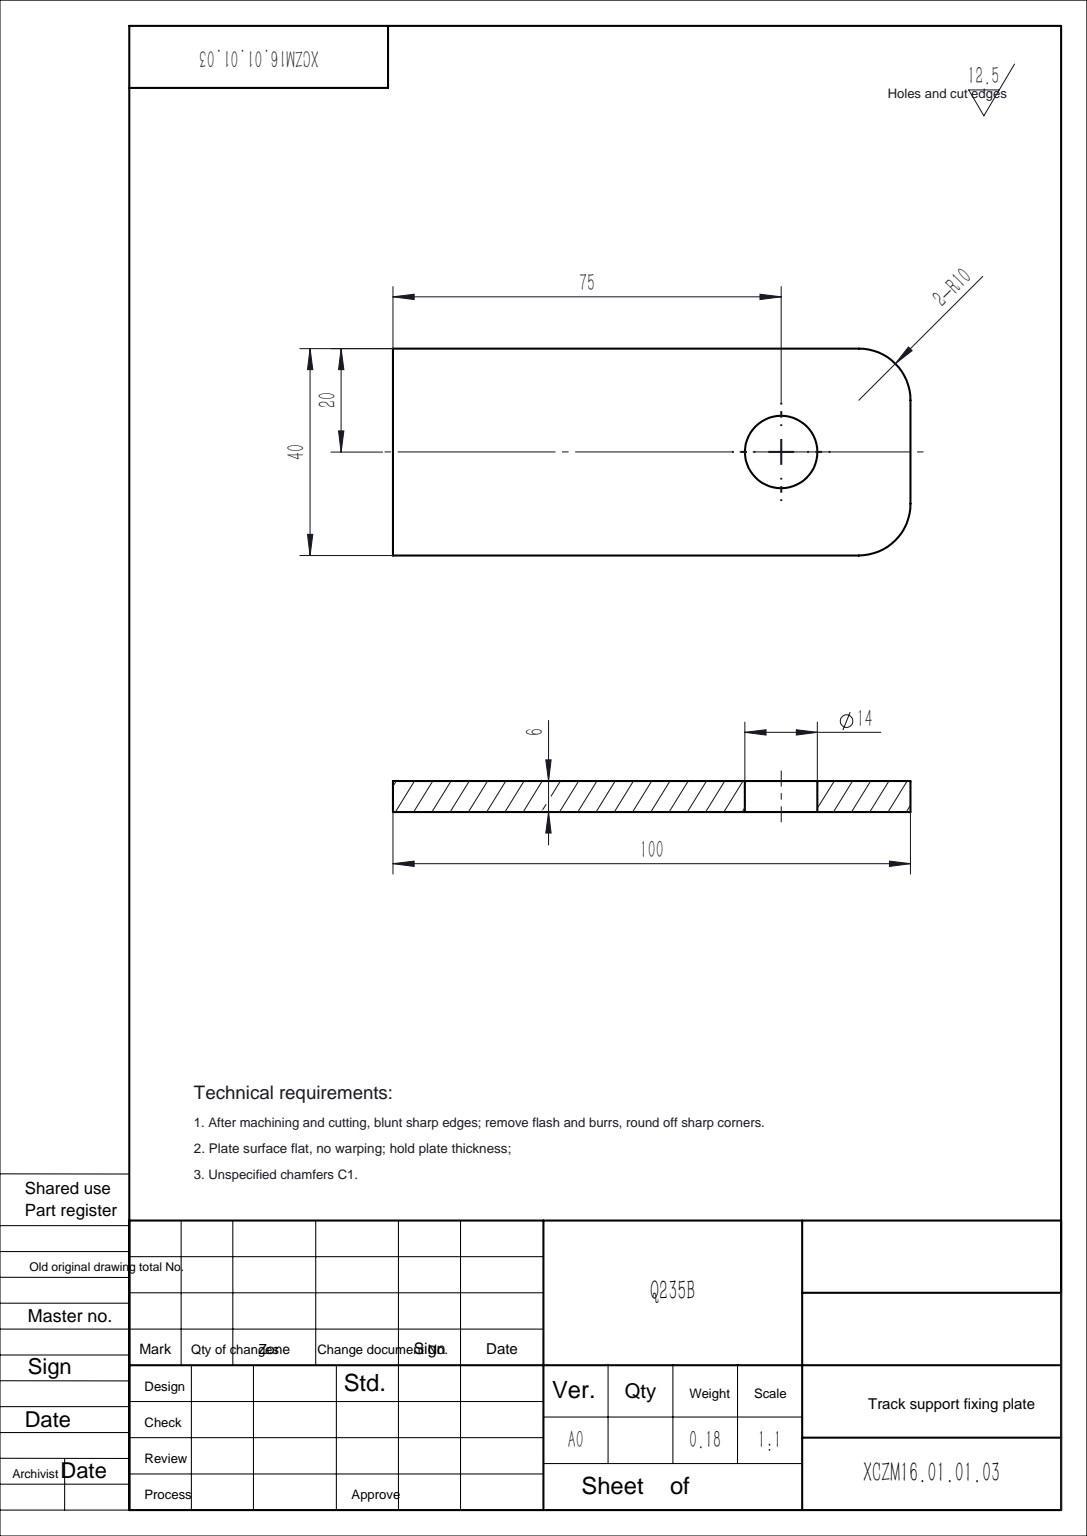
SolidWorks part; units mm, degrees
material "Q235B"
ref_plane "Front Plane" through (0, 0, 0) normal (0, 0, 1) x (1, 0, 0)
ref_plane "Top Plane" through (0, 0, 0) normal (0, 1, 0) x (1, 0, 0)
ref_plane "Right Plane" through (0, 0, 0) normal (1, 0, 0) x (0, 0, -1)
sketch "Sketch1" plane through (0, 0, 0) normal (0, 1, 0) x (1, 0, 0)
  line L1 (40, -20) -> (-50, -20)
  line L2 (50, -10) -> (50, 10)
  line L3 (40, 20) -> (-50, 20)
  line L4 (-50, -20) -> (-50, 20)
  line L5 (50, -20) -> (-50, 20) construction
  line L6 (50, 20) -> (-50, -20) construction
  arc A0 (40, -20) -> (50, -10) centre (40, -10) ccw
  arc A1 (50, 10) -> (40, 20) centre (40, 10) ccw
  circle A2 centre (25, 0) radius 7
  point P0 (0, 0)
  dimension "D3" = 10
  dimension "D4" = 14
  dimension "D1" = 40
  dimension "D2" = 100
  dimension "D5" = 75
extrude "Boss-Extrude1" add sketch "Sketch1" along normal blind 6
